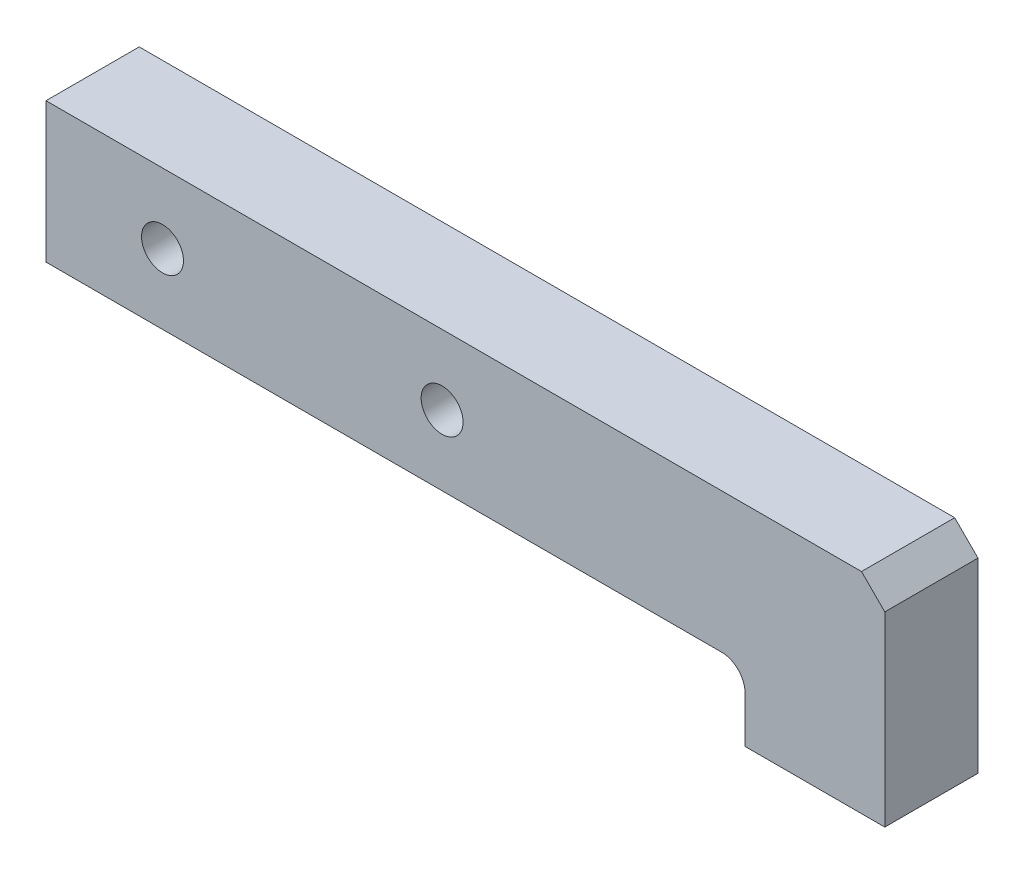
SolidWorks part; units mm, degrees
material "Q235A"
ref_plane "前视基准面" through (0, 0, 0) normal (0, 0, 1) x (1, 0, 0)
ref_plane "上视基准面" through (0, 0, 0) normal (0, 1, 0) x (1, 0, 0)
ref_plane "右视基准面" through (0, 0, 0) normal (1, 0, 0) x (0, 0, -1)
sketch "草图1" plane through (0, 0, 0) normal (0, 0, 1) x (1, 0, 0)
  line L1 (-90, 15) -> (90, 15)
  line L2 (-90, 15) -> (-90, -15)
  line L3 (-90, -15) -> (90, -15)
  line L4 (90, 15) -> (90, -15)
  line L5 (-90, 15) -> (90, -15) construction
  line L6 (-90, -15) -> (90, 15) construction
  point P0 (0, 0)
  dimension "D1" = 180
  dimension "400" = 30
extrude "凸台-拉伸1" add sketch "草图1" along normal blind 20
sketch "草图4" plane through (0, 0, 20) normal (0, 0, 1) x (1, 0, 0)
  line L0 (90, -15) -> (90, -30)
  line L1 (90, -30) -> (60, -30)
  line L2 (60, -30) -> (60, -15)
  line L3 (-90, -15) -> (90, -15) construction
  line L4 (90, 15) -> (-90, 15) construction
  line L5 (60, -15) -> (90, -15)
  dimension "D1" = 30
  dimension "D2" = 45
extrude "凸台-拉伸2" add sketch "草图4" against normal up to surface (20 mm away) contours L0 L1 L2 L5 up to face at (0, 0, 0)
fillet "圆角1" radius 5 1 edges at (60, -15, 10)
chamfer "倒角1" distance 5 angle 45 1 edges at (90, 15, 10)
hole_wizard "M8 螺纹孔2" positions "草图5" profile "草图6" tap size "M8" standard "GB"
sketch "草图5" plane through (0, -30, 0) normal (0, -1, 0) x (-1, 0, 0)
  line L0 (-75, 0) -> (-75, -10) construction
  line L1 (-60, 0) -> (-90, 0) construction
  line L2 (-75, -10) -> (-90, -10) construction
  line L3 (-90, 0) -> (-90, -20) construction
  point P0 (-75, -10)
sketch "草图6" plane through (75, -30, 10) normal (1, 0, 0) x (0, 0, -1)
  line L0 (0, 0) -> (0, 21.7929)
  line L1 (0, 21.7929) -> (3.4, 19.75)
  line L2 (3.4, 19.75) -> (3.4, 0)
  line L5 (3.4, 0) -> (0, 0)
  line L10 (0, 21.7929) -> (-3.4, 19.75) construction
  line L11 (0, -6.35) -> (0, 107.95) construction
  dimension "螺纹孔钻头直径" = 6.8
  dimension "螺纹孔钻头深度" = 19.75
  dimension "导头角度" = 118
cosmetic thread "孔螺蚊线1" parameters "D1"=16, "D2"=8
hole_wizard "打孔尺寸(%根据)内六角圆柱头螺钉的类型1" positions "草图7" profile "草图8" counterbore size "M8" standard "GB"
sketch "草图7" plane through (0, 0, 0) normal (0, 0, -1) x (-1, 0, 0)
  line L0 (90, 0) -> (-90, 0) construction
  line L1 (90, 15) -> (90, -15) construction
  line L2 (-90, -30) -> (-90, 10) construction
  point P9 (5, 0)
  point P11 (65, 0)
  dimension "D1" = 25
  dimension "D2" = 60
sketch "草图8" plane through (-65, 0, 0) normal (1, 0, 0) x (0, 1, 0)
  line L0 (0, 0) -> (0, 30.2039)
  line L1 (0, 30.2039) -> (4.5, 27.5)
  line L2 (4.5, 27.5) -> (4.5, 9)
  line L3 (4.5, 9) -> (7.5, 9)
  line L4 (7.5, 9) -> (7.5, 0)
  line L5 (7.5, 0) -> (0, 0)
  line L10 (0, 30.2039) -> (-4.5, 27.5) construction
  line L11 (0, -6.35) -> (0, 107.95) construction
  dimension "孔直径" = 9
  dimension "孔深度" = 27.5
  dimension "柱形沉头孔直径" = 15
  dimension "柱形沉头孔深度" = 9
  dimension "导头角度" = 118
